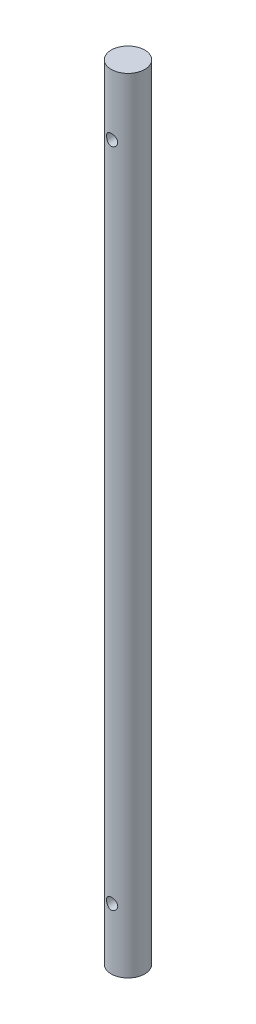
SolidWorks part; units mm, degrees
ref_plane "前视基准面" through (0, 0, 0) normal (0, 0, 1) x (1, 0, 0)
ref_plane "上视基准面" through (0, 0, 0) normal (0, 1, 0) x (1, 0, 0)
ref_plane "右视基准面" through (0, 0, 0) normal (1, 0, 0) x (0, 0, -1)
sketch "草图1" plane through (0, 0, 0) normal (0, 1, 0) x (1, 0, 0)
  circle A0 centre (0, 0) radius 6
  dimension "D1" = 12
extrude "凸台-拉伸1" add sketch "草图1" along normal mid plane 280
ref_plane "基准面1" through (0, 0, 11) normal (0, 0, 1) x (1, 0, 0)
sketch "草图3" plane through (0, 0, 11) normal (0, 0, 1) x (1, 0, 0)
  line L0 (0, -7.15) -> (0, 7.15) construction
  circle A0 centre (0, -118.2081) radius 2
  dimension "D1" = 4
  dimension "D2" = 118.2081
extrude "切除-拉伸1" cut sketch "草图3" against normal blind 60
mirror "镜向1" about plane through (0, 0, 0) normal (0, 1, 0) of "切除-拉伸1"
